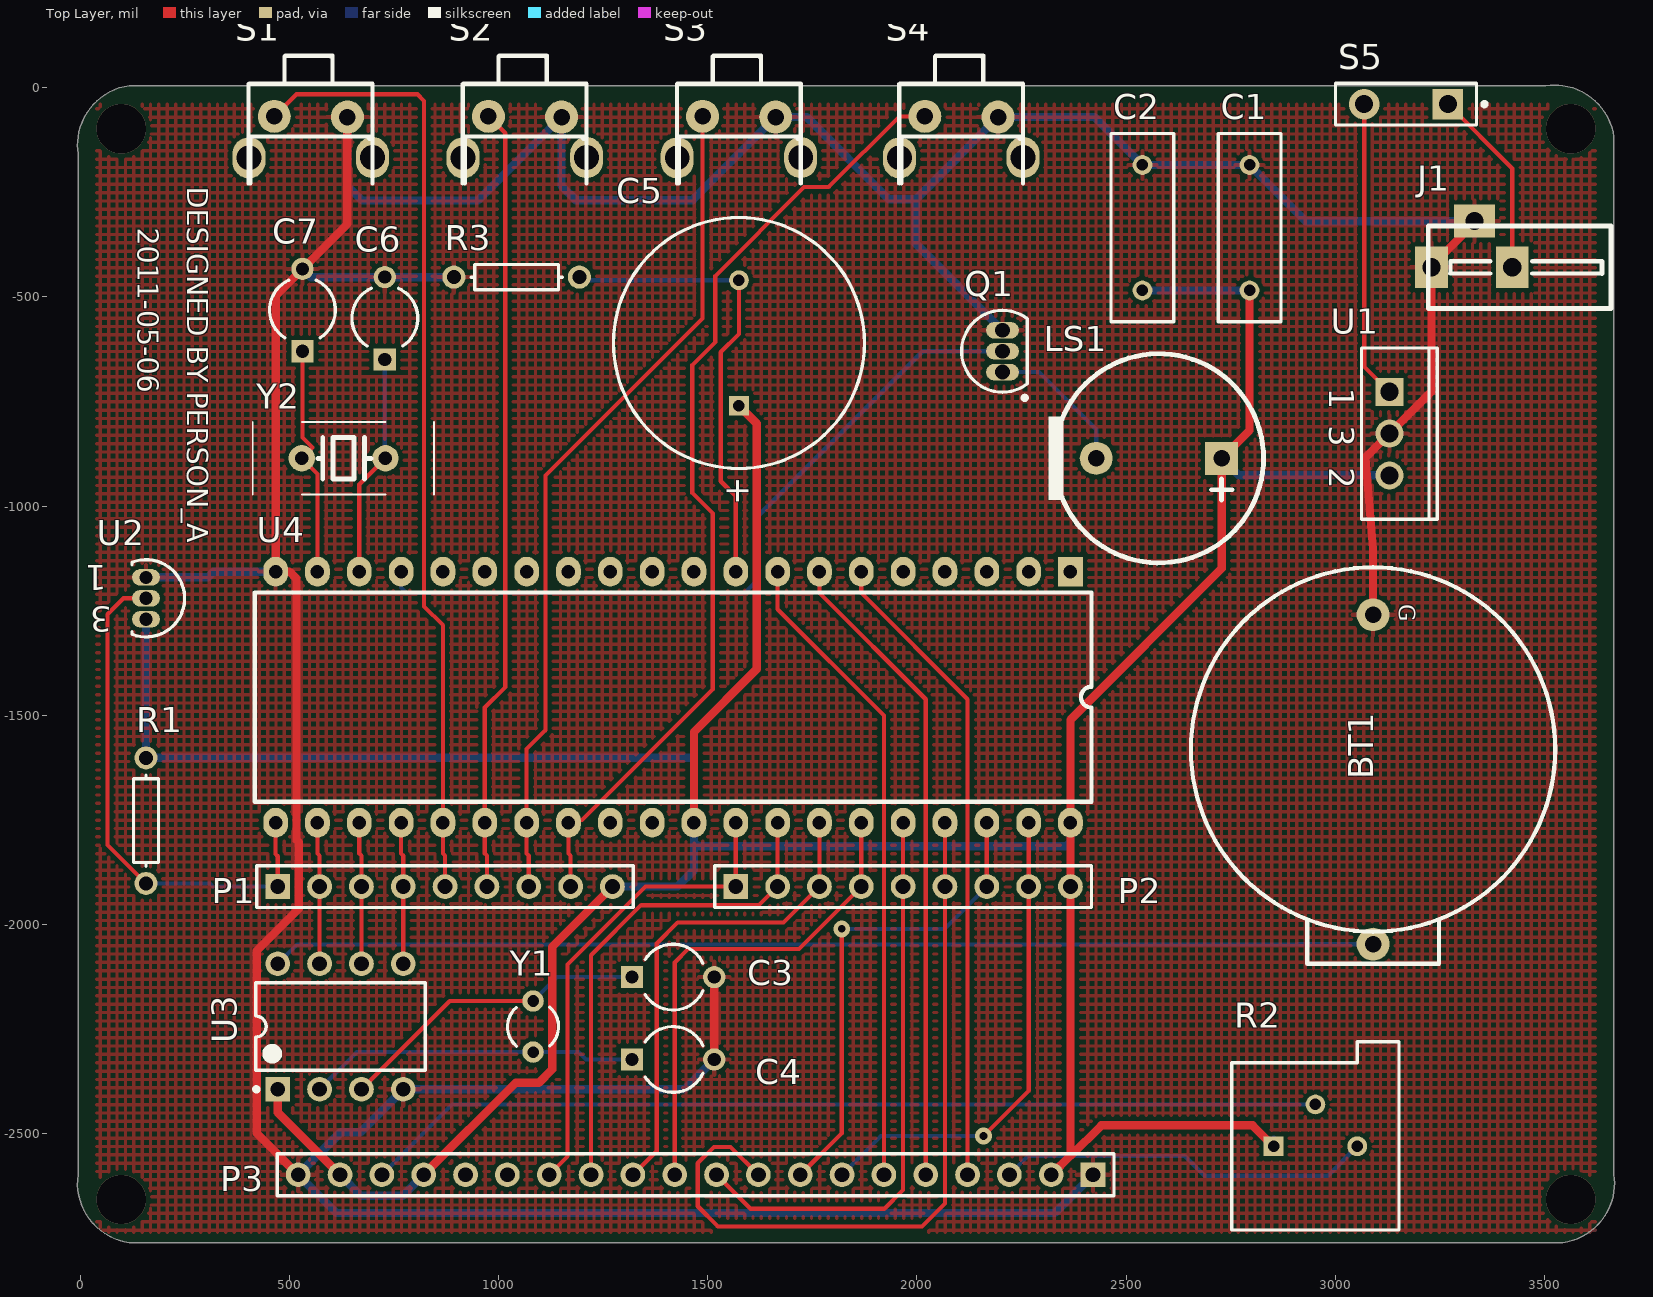
[diagram p0: Top Layer view]
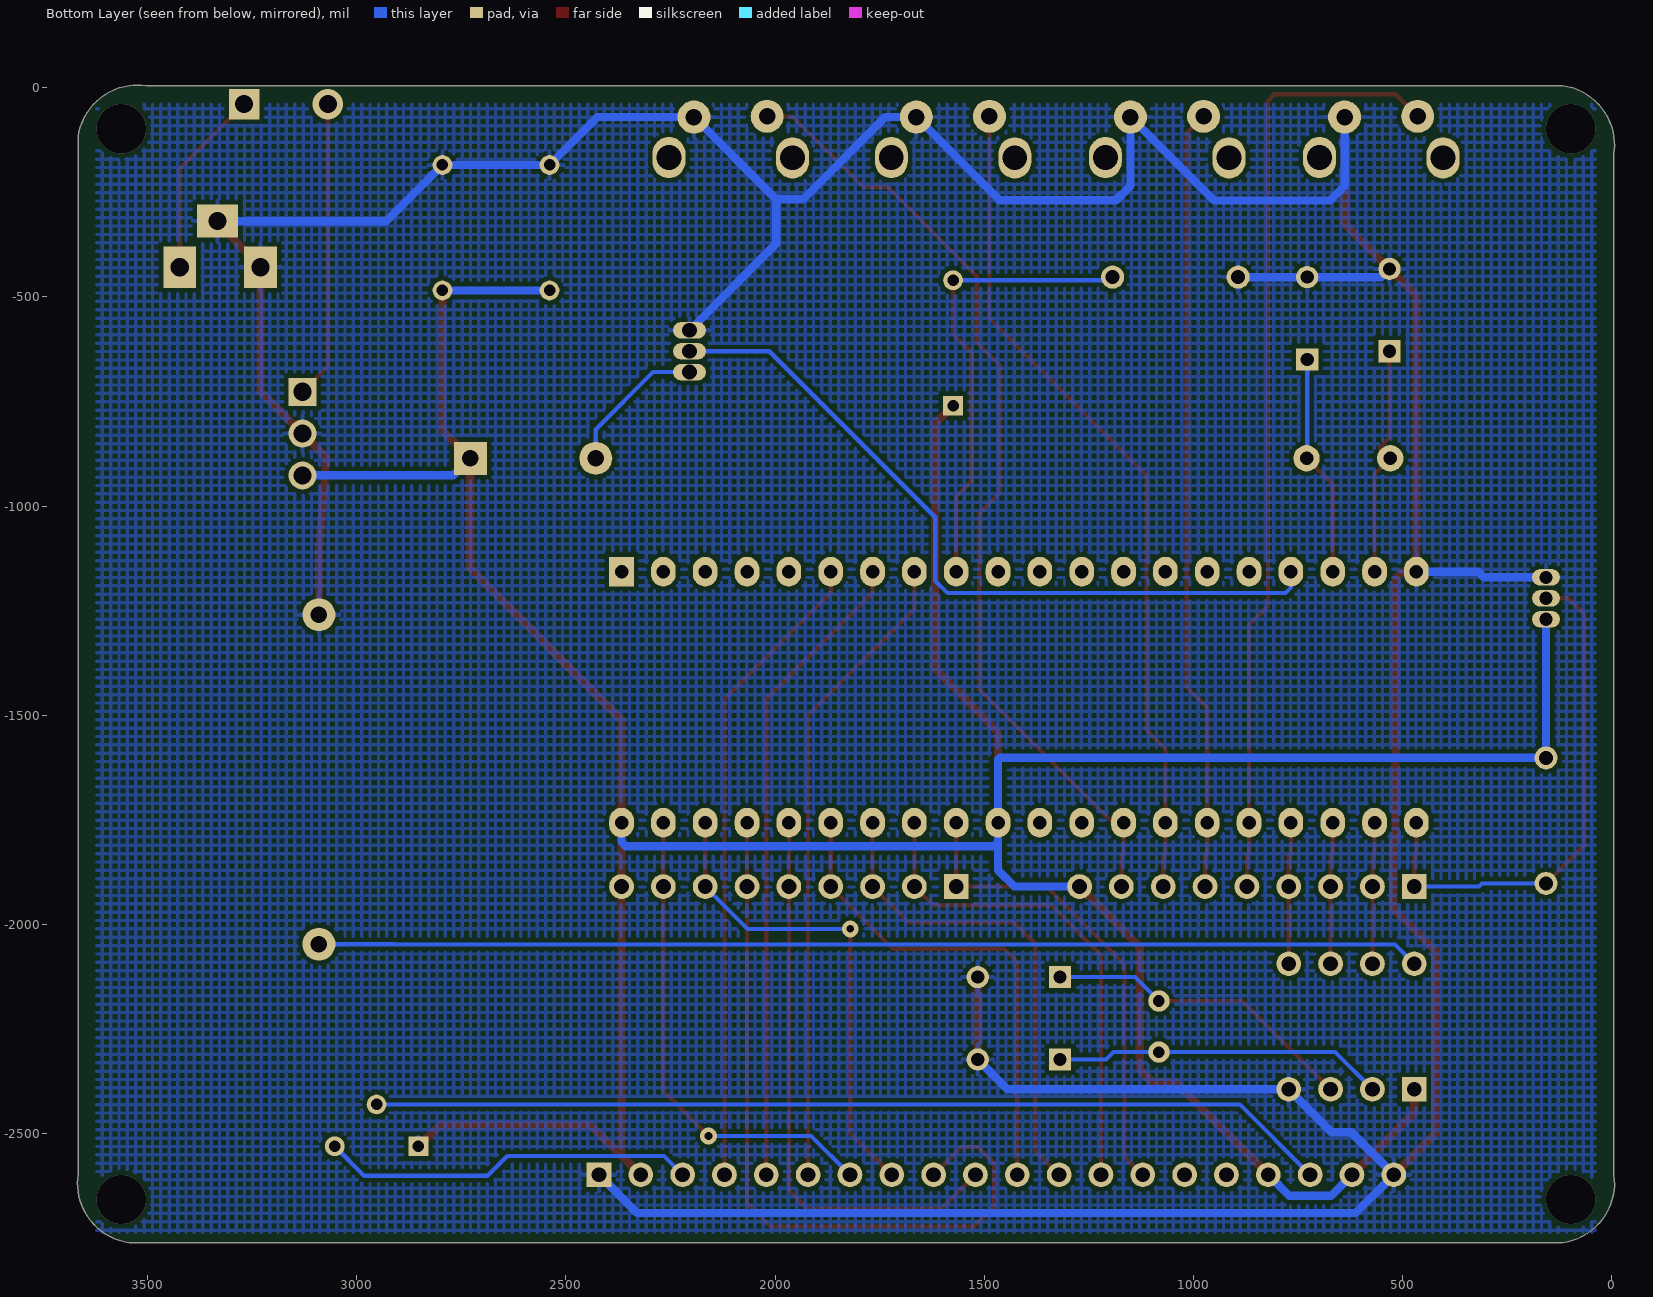
[diagram p1: Bottom Layer view, seen from below]
# Altium PCB MISC82171.PcbDoc
Units mil, origin at the board's own origin, x right, y up, seen from the top; angles counter-clockwise.
Board outline 3674.24 x 2767.33 mil, 2 copper layers (Top Layer, Bottom Layer); 28 components, 33 nets, 145 pads, 6 vias.

## Layer stack, top to bottom (the 12.6 mil dielectric is the usual default, probably not edited)
Top Layer: signal copper 1.4
Dielectric: dielectric 12.6, FR-4, Dk 4.8
Bottom Layer: signal copper 1.4

## Board outline
117.4,-2760.87 cw(c137.8,-2618.11) -5.01,-2598.07 -5.01,-157.83 cw(c137.8,-137.8) -4.96,-117.4 cw(c137.8,-137.8) 117.4,4.96 cw(c118.11,0) 118.11,5.01 3503.58,5.01 cw(c3523.62,-137.8) 3544.02,4.96 cw(c3523.62,-137.8) 3666.38,-117.4 cw(c3661.42,-118.11) 3666.43,-118.11 3666.43,-2598.07 cw(c3523.62,-2618.11) 3667.83,-2618.11 cw(c3523.62,-2618.11) 3666.38,-2638.5 cw(c3523.62,-2618.11) 3544.02,-2760.87 cw(c3543.31,-2755.91) 3543.31,-2760.92 118.11,-2760.92 cw(c118.11,-2755.91)

## Design rules (kind name [scope] priority, off if disabled: settings)
Clearance [All] p1: gap=10
HoleSize [All] p1: absolutevalues=TRUE maxlimit=139.37 minlimit=1 maxpercent=80.000 minpercent=20.000
MinimumSolderMaskSliver [All] p1: minsoldermaskwidth=2
PolygonConnect [All] p1: connectstyle=Relief reliefconductorwidth=10 reliefentries=4 polygonreliefangle="90 Angle"
RoutingTopology [All] p1: topology=Horizontal
RoutingVias [All] p1: holewidth=18 width=40 viastyle="Through Hole" minholewidth=38 minwidth=60 maxholewidth=28 maxwidth=50
SilkToSilkClearance [All] p1: silktosilkclearance=2
SilkscreenOverComponentPads [All] p1: minsilkscreentomaskgap=0
SolderMaskExpansion [All] p1: expansion=4
Width power [InNet('VCC') Or InNet('GND')] p1: maxlimit=30 minlimit=8 preferedwidth=20
Width [All] p2: maxlimit=20 minlimit=5 preferedwidth=10
23 further rules are at their usual default settings.

## Components (designator, comment, footprint, x,y, rotation, side; value= is the part's Value field where it differs from the comment)
BT1 "Battery" 3V电池 3090.55,-1653.54 r0 top
C1 "Cap" RAD-0.3 2795.28,-334.65 r270 top
C2 "Cap" RAD-0.3 2539.37,-334.65 r270 top
C3 "Cap2" CAPR5-4X5 1417.32,-2125.98 r0 top
C4 "Cap2" CAPR5-4X5 1417.32,-2322.83 r0 top
C5 "Cap Pol1" RB7.6-15 1574.8,-610.24 r270 top
C6 "Cap2" CAPR5-4X5 728.35,-551.18 r90 top
C7 "Cap2" CAPR5-4X5 531.5,-531.5 r90 top
J1 "PWR2.5" DC 3326.77,-374.02 r0 top
LS1 "Bell" BELL 2578.74,-885.83 r90 top
P1 "Header 9" HDR1X9 472.44,-1909.45 r0 top
P2 "Header 9" HDR1X9 1567.32,-1909.45 r0 top
P3 "Header 20" HDR1X20 2421.26,-2598.43 r180 top locked
Q1 "2N3906" TO-92A 2204.72,-629.92 r0 top
R1 "Res1" AXIAL-0.3 157.48,-1751.97 r270 top
R2 "RPot" VR4 2952.76,-2480.32 r0 top
R3 "Res1" AXIAL-0.3 1043.31,-452.76 r0 top
S1 "SW-PB" SW4 551.18,-118.11 r270 top
S2 "SW-PB" SW4 1062.99,-118.11 r270 top
S3 "SW-PB" SW4 1574.8,-118.11 r270 top
S4 "SW-PB" SW4 2106.3,-118.11 r270 top
S5 "SW-SPST" SPST-2 3169.29,-39.37 r180 top
U1 "L7805ACV" TO220ABN 3129.92,-826.77 r270 top
U2 "DS1820" PR35 157.48,-1220.47 r180 top
U3 "DS1302" DIP8 622.44,-2244.09 r90 top
U4 "AT89S52-33PC" DIP40 1417.32,-1456.69 r0 top
Y1 "XTAL" R38 1082.68,-2244.09 r0 top
Y2 "XTAL" XTAL2 629.92,-885.83 r180 top

## Footprints (in the part's own frame and the unit in brackets; to place one, negate y for a bottom-side part, rotate by r counter-clockwise, add the part's x,y. Pads: shape width x height; smd on the part's side, far side on the other; paste and mask are expansions set on the pad)
3V电池 [mm]
  round 2 hole 1: 1(0,-10) 2(0,10)
  silkscreen extent -11.06,-11.19 11.06,12.88
AXIAL-0.3 [mm] "Axial Device, Thru-Hole; 2 Leads; 0.3 in Pin Spacing"
  round 1.4 hole 0.85: 1(-3.81,0) 2(3.81,0)
  silkscreen extent -2.77,-0.76 2.77,0.76
BELL [mm]
  rect 2x2 hole 1: 1(0,-3.81)
  round 2 hole 1: 2(0,3.81)
  silkscreen extent -6.35,-6.35 6.35,6.7
CAPR5-4X5 [mm] "Capacitor; 2 Leads"
  rect 1.35x1.35 hole 0.8: 1(-2.5,0)
  round 1.35 hole 0.8: 2(2.5,0)
  silkscreen extent -1.69,-2 1.82,2
DC [mm]
  rect 2x2.5 hole 1.1: 1(2.45,-1.4) 2(-2.45,-1.4)
  rect 2.5x2 hole 1.1: 3(0.15,1.4)
  silkscreen extent -2.65,-3.9 8.45,1.1
DIP8 [mm] "DIP, 8-Leads, Row Spacing 7.62mm, Pitch 2.54mm, Body 9.65x6.35mm"
  rect 1.5x1.5 hole 0.9: 1(-3.81,3.81)
  round 1.5 hole 0.9: 2(-3.81,1.27) 3(-3.81,-1.27) 4(-3.81,-3.81) 5(3.81,-3.81) 6(3.81,-1.27) 7(3.81,1.27) 8(3.81,3.81)
  silkscreen extent -3.93,-5.15 2.65,5.23, body extent -3.6,-5.15 3.6,5.15, height 4.42
DIP40 [mm]
  rect 1.5x1.8 hole 0.82: 1(24.13,7.62)
  oval 1.5x1.8 hole 0.82: 2(21.59,7.62) 3(19.05,7.62) 4(16.51,7.62) 5(13.97,7.62) 6(11.43,7.62) 7(8.89,7.62) 8(6.35,7.62) 9(3.81,7.62) 10(1.27,7.62) 11(-1.27,7.62) 12(-3.81,7.62) 13(-6.35,7.62) 14(-8.89,7.62) 15(-11.43,7.62) 16(-13.97,7.62) 17(-16.51,7.62) 18(-19.05,7.62) 19(-21.59,7.62) 20(-24.13,7.62) 21(-24.13,-7.62) 22(-21.59,-7.62) 23(-19.05,-7.62) 24(-16.51,-7.62) 25(-13.97,-7.62) 26(-11.43,-7.62) 27(-8.89,-7.62) 28(-6.35,-7.62) 29(-3.81,-7.62) 30(-1.27,-7.62) 31(1.27,-7.62) 32(3.81,-7.62) 33(6.35,-7.62) 34(8.89,-7.62) 35(11.43,-7.62) 36(13.97,-7.62) 37(16.51,-7.62) 38(19.05,-7.62) 39(21.59,-7.62) 40(24.13,-7.62)
  silkscreen extent -25.4,-6.35 25.4,6.35
HDR1X9 [mm] "Connector; Header; 9 Position"
  rect 1.5x1.5 hole 0.9: 1(0,0)
  round 1.5 hole 0.9: 2(2.54,0) 3(5.08,0) 4(7.62,0) 5(10.16,0) 6(12.7,0) 7(15.24,0) 8(17.78,0) 9(20.32,0)
  silkscreen extent -1.27,-1.27 21.59,1.27
HDR1X20 [mm] "Connector; Header; 20 Position"
  rect 1.5x1.5 hole 0.9: 1(0,0)
  round 1.5 hole 0.9: 2(2.54,0) 3(5.08,0) 4(7.62,0) 5(10.16,0) 6(12.7,0) 7(15.24,0) 8(17.78,0) 9(20.32,0) 10(22.86,0) 11(25.4,0) 12(27.94,0) 13(30.48,0) 14(33.02,0) 15(35.56,0) 16(38.1,0) 17(40.64,0) 18(43.18,0) 19(45.72,0) 20(48.26,0)
  silkscreen extent -1.27,-1.27 49.53,1.27
PR35 [mm] "TO, Flat Index; 3 In-Line, Axial Leads; Body Dia. 4.6mm; Leads 0.56 x 0.51 mm (max)"
  oval 1.7x1 hole 0.8: 1(0,-1.27) 2(0,0) 3(0,1.27)
  silkscreen extent -2.34,-2.35 0.85,2.35
R38 [mm] "Crystal, Thru-Hole; 2 Leads; Body 3.1 x 8.2 mm (Dia.xH)"
  round 1.3 hole 0.7: 1(0,1.55) 2(0,-1.55)
  silkscreen extent -1.55,-1.19 1.55,1.17
RAD-0.3 [mm] "Radial Cap, Thru-Hole; 2 Leads; 0.3 in Pin Spacing"
  round 1.2 hole 0.7: 1(-3.81,0) 2(3.81,0)
  silkscreen extent -5.72,-1.9 5.71,1.91
RB7.6-15 [mm] "Polarized Capacitor (Radial); 2 Leads"
  rect 1.2x1.2 hole 0.7: 1(3.81,0)
  round 1.2 hole 0.7: 2(-3.81,0)
  silkscreen extent -7.62,-7.62 7.62,7.62
SPST-2 [mm] "Switch; 2 Leads"
  rect 1.85x1.85 hole 1.1: 1(-2.54,0)
  round 1.85 hole 1.1: 2(2.54,0)
  silkscreen extent -4.89,-1.27 4.28,1.27
SW4 [mm]
  oval 2.5x2 hole 1.5: 0(1.24,3.75) 0(1.26,-3.75)
  round 2 hole 1: 1(-1.22,2.23) 2(-1.26,-2.21)
  silkscreen extent -4.96,-3.77 2.82,3.75
TO220ABN [mm] "TO, Thru-Hole, Vertical, Heatsink Mounted; 3 In-Line Leads; Pitch 2.54 mm; Pin sequence 1, 3, 2"
  rect 1.7x1.7 hole 1.1: 1(-2.54,0)
  round 1.7 hole 1.1: 2(2.54,0) 3(0,0)
  silkscreen extent -5.2,-1.7 5.2,2.9
TO-92A [mm] "TO, Flat Index; 3 In-Line, Axial Leads; Body Dia. 4.5mm; Leads 0.51 x 0.48 mm (max)"
  oval 2x1 hole 0.9: 1(0,-1.27) 2(0,0) 3(0,1.27)
  silkscreen extent -2.48,-2.95 1.5,2.48, body extent -2.5,-2.5 1.5,2.5, height 6.86
VR4 [mm] "Thru-Hole; 3 Leads"
  rect 1.2x1.2 hole 0.7: 1(-2.54,-1.27)
  round 1.2 hole 0.7: 2(0,1.27) 3(2.54,-1.27)
  silkscreen extent -5.08,-6.35 5.08,5.08
XTAL2 [mm]
  round 1.6 hole 0.82: 1(2.54,0) 2(-2.54,0)
  silkscreen extent -5.49,-2.2 5.51,2.2

## Part data
BT1: "Multicell Batter"
C1 C2 C3 C4 C6 C7: "Capacitor"
C5: "Polarized Capacitor (Radial)"
J1: "Low Voltage Power Supply Connector"
LS1: "Electrical Bell"
P1 P2: "Header, 9-Pin"
P3: "Header, 20-Pin"
Q1: "PNP General Purpose Amplifier"
R1 R3: "Resistor"
R2: "Potentiometer"
S1 S2 S3 S4: "Switch"
S5: "Single-Pole, Single-Throw Switch"
U1: "Precision 1A Regulator"
U2: "1-Wire Digital Thermometer"
U3: "Trickle Charge Timekeeping Chip"
U4: "Atmel 8 Bit Micro 4.0-5.5V 33MHz 0-70 Deg C 40 PDIP (40P6) Package"
Y1 Y2: "Crystal Oscillator"

## Via types
v1: diameter 118.11, hole 118.11, Top Layer to Bottom Layer, 4 vias
v2: diameter 40, hole 18, Top Layer to Bottom Layer, 2 vias

## Nets (pads, with @x,y where several pads share a name; then routed paths per layer and width w, separated by ;. In a path a pad name is that pad's centre, name@x,y a point inside that pad or via, vN(x,y) a via of type N, cw(c..) or ccw(c..) an arc to the next point about the centre after c; other vN are vias at no path point)
E: P3.6 U4.8 | length 1546.9
  Top Layer w10: U4.8 1667.32,-1246.71 1921.26,-1500.65 P3.6
GND: BT1.2 C1.1 C2.1 C3.2 C4.2 C6.2 C7.2 J1.2 J1.3 P3.1 P3.20 Q1.3 R3.1 S1.1 S2.1 S3.1 S4.1 U1.3 U2.1 U3.4 U4.20 | length 11621.7
  Top Layer w20: P3.20 422.35,-2499.51 422.35,-2062.71 522.35,-1962.71 522.35,-1803.71 517.35,-1798.71 517.35,-1173.69 500.35,-1156.69 U4.20 467.32,-497.24 C7.2 638.98,-325.59 S1.1 ; C4.2 C3.2 ; BT1.2 3090.55,-1102.91 3072.35,-884.35 U1.3 3230.31,-726.38 J1.2 3230.31,-425.71 3332.68,-323.34 J1.3
  Bottom Layer w20: U2.1 305.35,-1170.47 319.13,-1156.69 U4.20 ; C7.2 551.18,-452.76 C6.2 R3.1 ; S1.1 638.98,-234.71 673.98,-269.71 951.16,-269.71 S2.1 1150.79,-234.71 1184.79,-268.71 1463.97,-268.71 S3.1 1736.83,-70.08 1933.46,-266.71 1997.46,-266.71 ; C4.2 1444.49,-2394.09 U3.4 669.83,-2496.71 622.98,-2496.71 P3.20 612.54,-2689.71 2329.98,-2689.71 P3.1 ; Q1.3 1997.46,-372.66 1997.46,-266.71 ; J1.3 2929.53,-318.9 C1.1 C2.1 2424.8,-70.08 S4.1 1997.46,-266.71
NetBT1_1: BT1.1 U3.8 | length 2637.5
  Bottom Layer w10: U3.8 518.83,-2047.71 2909.35,-2047.71 2909.81,-2047.24 BT1.1
NetC3_1: C3.1 U3.3 Y1.1 | length 757.5
  Top Layer w10: U3.3 883.46,-2183.07 Y1.1
  Bottom Layer w10: Y1.1 1139.76,-2125.98 C3.1
NetC4_1: C4.1 U3.2 Y1.2 | length 790.7
  Bottom Layer w10: U3.2 661.42,-2305.12 Y1.2 1191.35,-2305.12 1209.06,-2322.83 C4.1
NetC5_2: C5.2 R3.2 U4.9 | length 1103.4
  Top Layer w10: U4.9 1567.32,-976.68 1531.35,-940.71 1531.35,-632.16 1574.8,-588.71 C5.2
  Bottom Layer w10: R3.2@1200.79,-460.24 C5.2
NetC6_1: C6.1 U4.18 Y2.2 | length 533.7
  Top Layer w10: U4.18 667.32,-948.42 Y2.2
  Bottom Layer w10: C6.1 728.35,-884.25 Y2.2
NetC7_1: C7.1 U4.19 Y2.1 | length 563
  Top Layer w10: C7.1 531.5,-835.83 555.71,-860.04 Y2.1 567.32,-923.23 U4.19
NetJ1_1: J1.1 S5.1 | length 453.5
  Top Layer w10: S5.1 3423.23,-193.31 J1.1
NetLS1_2: LS1.2 Q1.1 | length 350
  Bottom Layer w10: Q1.1 2292.35,-679.92 2428.74,-816.31 LS1.2
NetP1_1: P1.1 R1.2 U2.2 U4.21 | length 1262.3
  Top Layer w10: R1.2 65.35,-1809.83 65.35,-1258.71 103.58,-1220.47 U2.2 ; U4.21 467.32,-1832.01 472.44,-1837.13 P1.1
  Bottom Layer w10: R1.2 310.35,-1901.97 317.83,-1909.45 P1.1
NetP1_2: P1.2 U3.7 U4.22 | length 339.5
  Top Layer w10: U4.22 567.32,-1830.59 572.44,-1835.71 P1.2 U3.7
NetP1_3: P1.3 U3.6 U4.23 | length 339.5
  Top Layer w10: U4.23 667.32,-1830.59 672.44,-1835.71 P1.3 U3.6
NetP1_4: P1.4 U3.5 U4.24 | length 339.5
  Top Layer w10: U4.24 767.32,-1830.59 772.44,-1835.71 P1.4 U3.5
NetP2_1: P2.1 P3.14 U4.32 | length 1152.9
  Top Layer w10: P3.14 1165.35,-2554.34 1165.35,-2095.71 1351.61,-1909.45 P2.1 U4.32
NetP2_2: P2.2 P3.13 U4.33 | length 1191.5
  Top Layer w10: P3.13 1221.26,-2073.79 1341.08,-1953.98 1622.79,-1953.98 P2.2 U4.33
NetP2_3: P2.3 P3.12 U4.34 | length 1174.5
  Top Layer w10: P3.12 1378.3,-2541.38 1378.3,-2045.8 1428.35,-1995.75 1681.02,-1995.75 P2.3 U4.34
NetP2_4: P2.4 P3.11 U4.35 | length 1181.6
  Top Layer w10: P3.11 1421.26,-2090.71 1453.26,-2058.71 1718.06,-2058.71 P2.4 U4.35
NetP2_5: P2.5 P3.10 U4.36 | length 1376.4
  Top Layer w10: P3.10 1602.54,-2679.71 1922.32,-2679.71 1967.32,-2634.71 P2.5 U4.36
NetP2_6: P2.6 P3.9 U4.37 | length 1835.4
  Top Layer w10: P3.9 1554.54,-2531.71 1515.35,-2531.71 1476.35,-2570.71 1476.35,-2673.71 1524.35,-2721.71 2012.32,-2721.71 2067.32,-2666.71 P2.6 U4.37
NetP2_7: P2.7 P3.8 U4.38 | length 1170.4
  Top Layer w10: P3.8 1820.35,-2499.34 v2(1820.35,-2010.71) ; P2.7 U4.38
  Bottom Layer w10: v2(1820.35,-2010.71) 2066.06,-2010.71 P2.7
NetP2_8: P2.8 P3.7 U4.39 | length 1170.2
  Top Layer w10: v2(2159.35,-2505.71) 2267.32,-2397.73 P2.8 U4.39
  Bottom Layer w10: P3.7 1913.98,-2505.71 v2(2159.35,-2505.71)
NetP3_3: P3.3 R2.3 | length 898.6
  Bottom Layer w10: P3.3 2265.98,-2553.71 2640.35,-2553.71 2687.35,-2600.71 2982.36,-2600.71 R2.3
NetP3_18: P3.18 R2.2 | length 2301.1
  Bottom Layer w10: P3.18 889.37,-2430.31 R2.2
NetQ1_2: Q1.2 U4.17 | length 1809.2
  Bottom Layer w10: U4.17 767.32,-1194.71 780.32,-1207.71 1588.35,-1207.71 1617.35,-1178.71 1617.35,-1026.71 2014.13,-629.92 Q1.2
NetS5_2: S5.2 U1.1 | length 712.5
  Top Layer w10: S5.2 3069.29,-666.14 U1.1
RS: P3.4 U4.6 | length 1546.9
  Top Layer w10: U4.6 1867.32,-1207.71 2121.26,-1461.65 P3.4
RW: P3.5 U4.7 | length 1546.9
  Top Layer w10: U4.7 1767.32,-1207.71 2021.26,-1461.65 P3.5
SW0: P1.5 S1.2 U4.25 | length 2285.2
  Top Layer w10: S1.2 516.97,-15.71 806.35,-15.71 822.35,-31.71 822.35,-1239.71 867.32,-1284.68 U4.25 867.32,-1830.59 872.44,-1835.71 P1.5
SW1: P1.6 S2.2 U4.26 | length 1880.1
  Top Layer w10: P1.6 972.44,-1835.71 967.32,-1830.59 U4.26 967.32,-1481.71 1016.35,-1432.68 1016.35,-108.86 S2.2
SW2: P1.7 S3.2 U4.27 | length 2017.2
  Top Layer w10: P1.7 1072.44,-1835.71 1067.32,-1830.59 U4.27 1067.32,-1580.73 1112.35,-1535.71 1112.35,-927.16 1487.79,-551.71 S3.2
SW3: P1.8 S4.2 U4.28 | length 2325.5
  Top Layer w10: P1.8 1172.44,-1835.71 1167.32,-1830.59 U4.28 1167.32,-1750.71 1199.35,-1750.71 1512.35,-1437.71 1512.35,-1017.71 1463.35,-968.71 1463.35,-662.71 1518.35,-607.71 1518.35,-449.71 1730.35,-237.71 1789.35,-237.71 1958.55,-68.5 S4.2
VCC: C1.2 C2.2 C5.1 LS1.1 P1.9 P2.9 P3.2 P3.17 P3.19 R1.1 R2.1 U1.2 U2.3 U3.1 U4.31 U4.40 | length 9098.9
  Top Layer w20: U3.1 472.44,-2449.6 P3.19 ; P3.17 1040.98,-2378.71 1096.35,-2378.71 1128.35,-2346.71 1128.35,-2053.54 P1.9 ; U4.31 1467.32,-1539.73 1617.35,-1389.71 1617.35,-802.78 C5.1 ; P3.2 2367.32,-2552.36 P2.9 U4.40 2367.32,-1510.73 2728.74,-1149.31 LS1.1 2795.28,-819.29 C1.2 ; 2368.9,-2552.36 2440.94,-2480.32 2802.76,-2480.32 R2.1
  Bottom Layer w20: U2.3 R1.1 1463.58,-1601.97 1467.32,-1605.71 U4.31 1467.32,-1803.68 ; P3.19 671.54,-2648.71 770.98,-2648.71 P3.17 ; P1.9 1428.35,-1909.45 1467.32,-1870.47 1467.32,-1803.68 ; U4.40 2367.32,-1802.71 2357.32,-1812.71 1476.35,-1812.71 1467.32,-1803.68 ; C2.2 C1.2 ; LS1.1 2769.69,-926.77 U1.2 ; R2.1 R2.1@2852.76,-2514.71
pads on no net: P3.15 P3.16 S1.0 S2.0 S3.0 S4.0 U4.1 U4.2 U4.3 U4.4 U4.5 U4.10 U4.11 U4.12 U4.13 U4.14 U4.15 U4.16 U4.29 U4.30
copper on no net:
  other v1: 98.43,-2657.48 3562.99,-2657.48 98.43,-98.43 3562.99,-98.43

## Polygon pours and split planes (outlines as drawn)
GND on Top Layer "Top Overlay-No Net" (hatched 90Degree grid 20 track 8, pour order 2): 39.37,-39.37 3622.05,-39.37 3622.05,-2736.22 59.06,-2736.22 39.37,-2716.54 39.37,-39.37
GND on Bottom Layer "Top Overlay-No Net" (hatched 90Degree grid 20 track 8, pour order 4): 39.37,-39.37 3622.05,-39.37 3622.05,-2736.22 39.37,-2736.22 39.37,-39.37

## Other copper
Bottom Layer:
  text "DS1302" at 1594.49,-4330.71 h30 r270
  text "DS1302" at 1614.17,-4330.71 h30 r270
  text "DS1302" at 1614.17,-4330.71 h30 r270

## Silkscreen, mask and mechanical layers (free items; w line width, h text height)
Top Overlay:
  text "DESIGNED BY PERSON_A" at 255.91,-236.22 h50 r270
  text "2011-05-06" at 137.8,-334.65 h50 r270